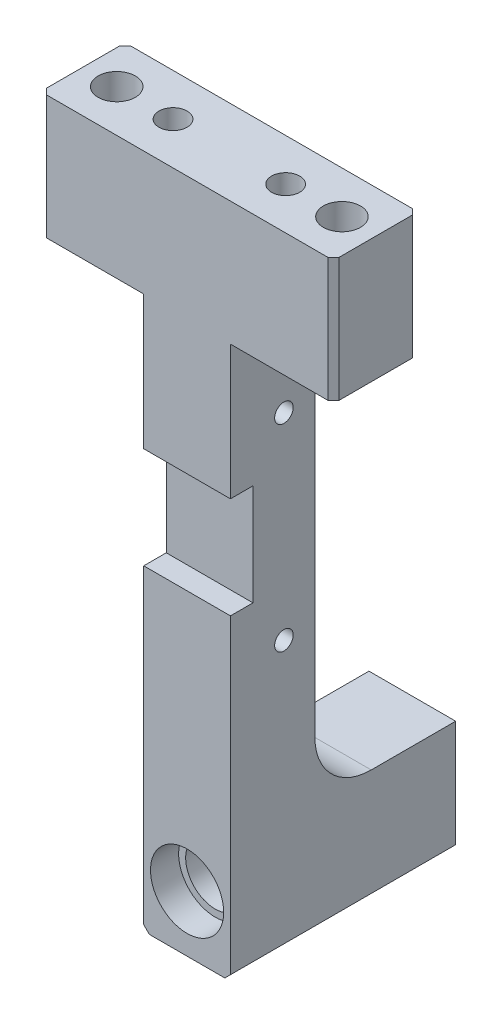
SolidWorks part; units mm, degrees
material "45"
ref_plane "Front Plane" through (0, 0, 0) normal (0, 0, 1) x (1, 0, 0)
ref_plane "Top Plane" through (0, 0, 0) normal (0, 1, 0) x (1, 0, 0)
ref_plane "Right Plane" through (0, 0, 0) normal (1, 0, 0) x (0, 0, -1)
sketch "Sketch1" plane through (0, 0, 0) normal (0, 0, 1) x (1, 0, 0)
  line L1 (-26, 60) -> (26, 60)
  line L2 (-26, 60) -> (-26, -60)
  line L3 (-26, -60) -> (26, -60)
  line L4 (26, 60) -> (26, -60)
  line L5 (-26, 60) -> (26, -60) construction
  line L6 (-26, -60) -> (26, 60) construction
  point P0 (0, 0)
  dimension "D1" = 120
  dimension "D2" = 52
extrude "Boss-Extrude1" add sketch "Sketch1" along normal mid plane 15
sketch "Sketch3" plane through (0, 0, 7.5) normal (0, 0, 1) x (1, 0, 0)
  line L0 (-26, -60) -> (26, -60) construction
  circle A0 centre (0, -50) radius 6.5
  dimension "D1" = 13
  dimension "D2" = 10
extrude "Cut-Extrude1" [suppressed] cut sketch "Sketch3" against normal blind 5
sketch "Sketch4" [suppressed] plane through (0, 0, 7.5) normal (0, 0, 1) x (1, 0, 0)
  circle A0 centre (0, -50) radius 5.25
  dimension "D1" = 10.5
extrude "Cut-Extrude2" [suppressed] cut sketch "Sketch4" against normal through all
sketch "Sketch5" [suppressed] plane through (0, 0, -7.5) normal (0, 0, -1) x (-1, 0, 0)
  circle A0 centre (0, -50) radius 6.5
  dimension "D1" = 13
extrude "Cut-Extrude3" [suppressed] cut sketch "Sketch5" against normal blind 5
sketch "Sketch8" plane through (0, 0, 7.5) normal (0, 0, 1) x (1, 0, 0)
  line L0 (-26, -60) -> (26, -60) construction
  line L1 (-26, 38) -> (-7.7, 38)
  line L2 (-26, 38) -> (-26, -60)
  line L3 (-26, -60) -> (-7.7, -60)
  line L4 (-7.7, 38) -> (-7.7, -60)
  line L5 (-26, 38) -> (-7.7, -60) construction
  line L6 (-26, -60) -> (-7.7, 38) construction
  line L7 (-26, 60) -> (-26, -60) construction
  line L8 (26, 60) -> (-26, 60) construction
  point P0 (-16.85, -11)
  dimension "D1" = 22
  dimension "D2" = 18.3
extrude "Cut-Extrude4" cut sketch "Sketch8" against normal through all
mirror "Mirror1" about plane through (0, 0, 0) normal (1, 0, 0) of "Cut-Extrude4"
hole_wizard "Ø6.6 (6.6) Diameter Hole1" positions "Sketch9" profile "Sketch10" hole size "Ø6.6" standard "ISO" end condition through all
sketch "Sketch9" plane through (0, 60, 0) normal (0, 1, 0) x (1, 0, 0)
  line L0 (0, 0) -> (0, 14.4083) construction
  line L3 (26, -7.5) -> (26, 7.5) construction
  point P0 (-20, 0)
  point P2 (20, 0)
  dimension "D1" = 6
sketch "Sketch10" plane through (-20, 60, 0) normal (1, 0, 0) x (0, 0, 1)
  line L0 (0, 0) -> (0, 120)
  line L1 (0, 120) -> (3.3, 120)
  line L2 (3.3, 120) -> (3.3, 0)
  line L5 (3.3, 0) -> (0, 0)
  line L11 (0, -6.35) -> (0, 107.95) construction
  dimension "通孔孔直径" = 6.6
  dimension "通孔孔深度" = 120
chamfer "Chamfer1" distance 1 angle 45 6 edges at (7.7, -60, 0) (-7.7, -60, 0) (-26, 49, -7.5) (-26, 49, 7.5) (26, 49, -7.5) (26, 49, 7.5)
hole_wizard "Blind Pin Hole1 size mm" positions "Sketch11" profile "Sketch12" hole size "Ø5.0" standard "ISO"
sketch "Sketch11" plane through (0, 60, 0) normal (0, 1, 0) x (1, 0, 0)
  line L0 (0, 0) -> (0, 19.0932) construction
  point P0 (-10, 0)
  point P2 (10, 0)
  dimension "D1" = 20
sketch "Sketch12" plane through (-10, 60, 0) normal (1, 0, 0) x (0, 0, 1)
  line L0 (0, 0) -> (0, 12.5022)
  line L1 (0, 12.5022) -> (2.5, 11)
  line L2 (2.5, 11) -> (2.5, 0)
  line L5 (2.5, 0) -> (0, 0)
  line L10 (0, 12.5022) -> (-2.5, 11) construction
  line L11 (0, -6.35) -> (0, 107.95) construction
  dimension "孔直径" = 5
  dimension "孔深度" = 11
  dimension "导头角度" = 118
sketch "Sketch13" plane through (0, 0, -7.5) normal (0, 0, -1) x (-1, 0, 0)
  line L0 (-7.7, -40) -> (7.7, -40)
  line L1 (-7.7, -59) -> (-7.7, 38) construction
  line L2 (7.7, -59) -> (7.7, 38) construction
  line L3 (7.7, -40) -> (7.7, -59)
  line L4 (7.7, -59) -> (6.7, -60)
  line L5 (6.7, -60) -> (-6.7, -60)
  line L6 (-6.7, -60) -> (-7.7, -59)
  line L7 (-7.7, -59) -> (-7.7, -40)
  dimension "D1" = 20
extrude "Boss-Extrude2" add sketch "Sketch13" along normal blind 25
fillet "Fillet1" radius 10 1 edges at (0, -40, -7.5)
sketch "Sketch14" plane through (0, 0, 7.5) normal (0, 0, 1) x (1, 0, 0)
  line L0 (0, -60) -> (0, -50) construction
  line L1 (-6.7, -60) -> (6.7, -60) construction
  circle A0 centre (0, -50) radius 5.25
  dimension "D1" = 10.5
  dimension "D2" = 10
extrude "Cut-Extrude5" cut sketch "Sketch14" against normal through all
sketch "Sketch15" plane through (0, 0, 7.5) normal (0, 0, 1) x (1, 0, 0)
  circle A0 centre (0, -50) radius 6.5
  dimension "D1" = 13
extrude "Cut-Extrude6" cut sketch "Sketch15" against normal blind 5
sketch "Sketch16" plane through (0, 0, -32.5) normal (0, 0, -1) x (-1, 0, 0)
  circle A0 centre (0, -50) radius 6.5
  dimension "D1" = 13
extrude "Cut-Extrude7" cut sketch "Sketch16" against normal blind 5
sketch "Sketch17" plane through (7.7, 0, 0) normal (1, 0, 0) x (0, 0, -1)
  line L0 (-7.5, -59) -> (-7.5, 38) construction
  line L1 (-7.5, 14.2) -> (-3.5, 14.2)
  line L2 (-7.5, 14.2) -> (-7.5, -3.8)
  line L3 (-7.5, -3.8) -> (-3.5, -3.8)
  line L4 (-3.5, 14.2) -> (-3.5, -3.8)
  line L7 (-6.5, 60) -> (6.5, 60) construction
  point P6 (-3.5, 5.2)
  dimension "D1" = 54.8
  dimension "D2" = 18
  dimension "D3" = 4
extrude "Cut-Extrude8" cut sketch "Sketch17" against normal through all
sketch "Sketch18" plane through (7.7, 0, 0) normal (1, 0, 0) x (0, 0, -1)
  line L0 (7.5, -30) -> (7.5, 38) construction
  line L1 (7.5, -8.8) -> (-3.5, -8.8)
  line L2 (7.5, -8.8) -> (7.5, 19.2)
  line L3 (7.5, 19.2) -> (-3.5, 19.2)
  line L4 (-3.5, -8.8) -> (-3.5, 19.2)
  line L6 (-3.5, 5.2) -> (7.5, 5.2) construction
  line L7 (-3.5, -3.8) -> (-3.5, 14.2) construction
  dimension "D1" = 11
  dimension "D2" = 28
extrude "Boss-Extrude3" [suppressed] add sketch "Sketch18" along normal blind 22
hole_wizard "M4 Tapped Hole1" positions "Sketch19" profile "Sketch20" tap size "M4" standard "GB"
sketch "Sketch19" plane through (7.7, 0, 0) normal (1, 0, 0) x (0, 0, -1)
  line L0 (-6.5, 60) -> (6.5, 60) construction
  line L1 (7.5, -30) -> (7.5, 38) construction
  point P0 (2, 22.7)
  point P2 (2, -12.3)
  dimension "D1" = 37.3
  dimension "D2" = 35
  dimension "D3" = 5.5
sketch "Sketch20" plane through (7.7, 22.7, -2) normal (0, 1, 0) x (0, 0, -1)
  line L0 (0, 0) -> (0, 11.0914)
  line L1 (0, 11.0914) -> (1.65, 10.1)
  line L2 (1.65, 10.1) -> (1.65, 0)
  line L5 (1.65, 0) -> (0, 0)
  line L10 (0, 11.0914) -> (-1.65, 10.1) construction
  line L11 (0, -6.35) -> (0, 107.95) construction
  dimension "螺纹孔钻头直径" = 3.3
  dimension "螺纹孔钻头深度" = 10.1
  dimension "导头角度" = 118
cosmetic thread "Cosmetic Thread1" parameters "D1"=8, "D2"=4
cosmetic thread "Cosmetic Thread2" parameters "D1"=8, "D2"=4
